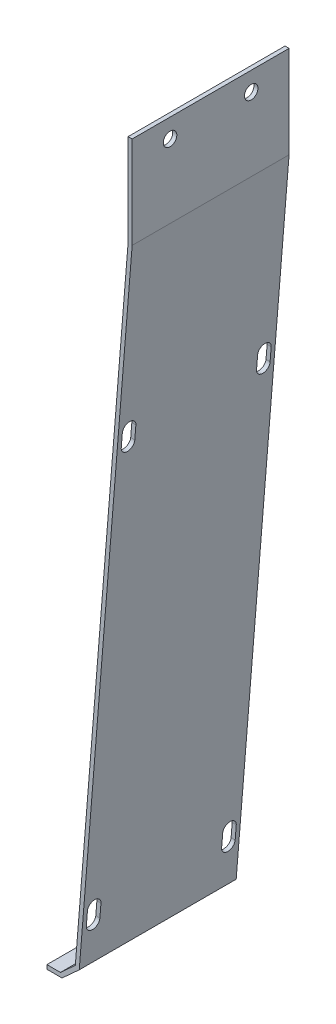
SolidWorks part; units mm, degrees
material "SPCC"
ref_plane "Front Plane" through (0, 0, 0) normal (0, 0, 1) x (1, 0, 0)
ref_plane "Top Plane" through (0, 0, 0) normal (0, 1, 0) x (1, 0, 0)
ref_plane "Right Plane" through (0, 0, 0) normal (1, 0, 0) x (0, 0, -1)
sketch "Sketch1" plane through (0, 0, 0) normal (0, 0, 1) x (1, 0, 0)
  line L0 (0, 0) -> (0, -34)
  line L1 (0, -34) -> (-19.5, -275)
  line L2 (-19.5, -275) -> (-25, -280)
  line L3 (-25, -280) -> (-30, -280)
  line L4 (0, 0) -> (-35.0092, 0) construction
  line L5 (-30, -280) -> (-30, 40.4183) construction
  dimension "D1" = 30
  dimension "D2" = 34
  dimension "D3" = 280
  dimension "D4" = 10.5
  dimension "D5" = 5
  dimension "D6" = 5
extrude "Extrude-Thin2" add sketch "Sketch1" along normal blind 58 thin thin type one direction reverse wall 1.5
sketch "Sketch2" plane through (1.5, 0, 0) normal (1, 0, 0) x (0, 0, -1)
  line L0 (-14, -7) -> (-44, -7) construction
  line L1 (0, 0) -> (0, -34.0606) construction
  line L2 (-58, 0) -> (-58, -34.0606) construction
  line L3 (-58, 0) -> (0, 0) construction
  circle A0 centre (-14, -7) radius 2.5
  circle A1 centre (-44, -7) radius 2.5
  dimension "D1" = 5
  dimension "D2" = 14
  dimension "D3" = 14
  dimension "D4" = 7
extrude "Cut-Extrude1" cut sketch "Sketch2" against normal blind 10
sketch "Sketch3" plane through (4.2283, -0.3421, 0) normal (0.9967, -0.0806, 0) x (0, 0, -1)
  line L0 (-54, -97.379) -> (-54, -102.379) construction
  line L1 (-51.5, -97.379) -> (-51.5, -102.379)
  line L2 (-56.5, -97.379) -> (-56.5, -102.379)
  line L3 (-58, -33.8287) -> (-58, -276.2692) construction
  line L4 (-58, 0.121) -> (0, 0.121) construction
  line L6 (-54, -262.379) -> (-54, -257.379) construction
  line L7 (-51.5, -262.379) -> (-51.5, -257.379)
  line L8 (-56.5, -262.379) -> (-56.5, -257.379)
  arc A0 (-51.5, -97.379) -> (-56.5, -97.379) centre (-54, -97.379) ccw
  arc A1 (-56.5, -102.379) -> (-51.5, -102.379) centre (-54, -102.379) ccw
  arc A2 (-51.5, -262.379) -> (-56.5, -262.379) centre (-54, -262.379) cw
  arc A3 (-56.5, -257.379) -> (-51.5, -257.379) centre (-54, -257.379) cw
  point P2 (-54, -99.879)
  point P15 (-54, -259.879)
  dimension "D1" = 5
  dimension "D2" = 4
  dimension "D3" = 5
  dimension "D4" = 100
  dimension "D5" = 260
  dimension "D6" = 5
  dimension "D7" = 4
  dimension "D8" = 5
extrude "Cut-Extrude2" cut sketch "Sketch3" against normal blind 10
ref_plane "Plane1" through (0, 0, 29) normal (0, 0, 1) x (1, 0, 0)
mirror "Mirror1" about plane through (0, 0, 29) normal (0, 0, 1) of "Cut-Extrude2"
